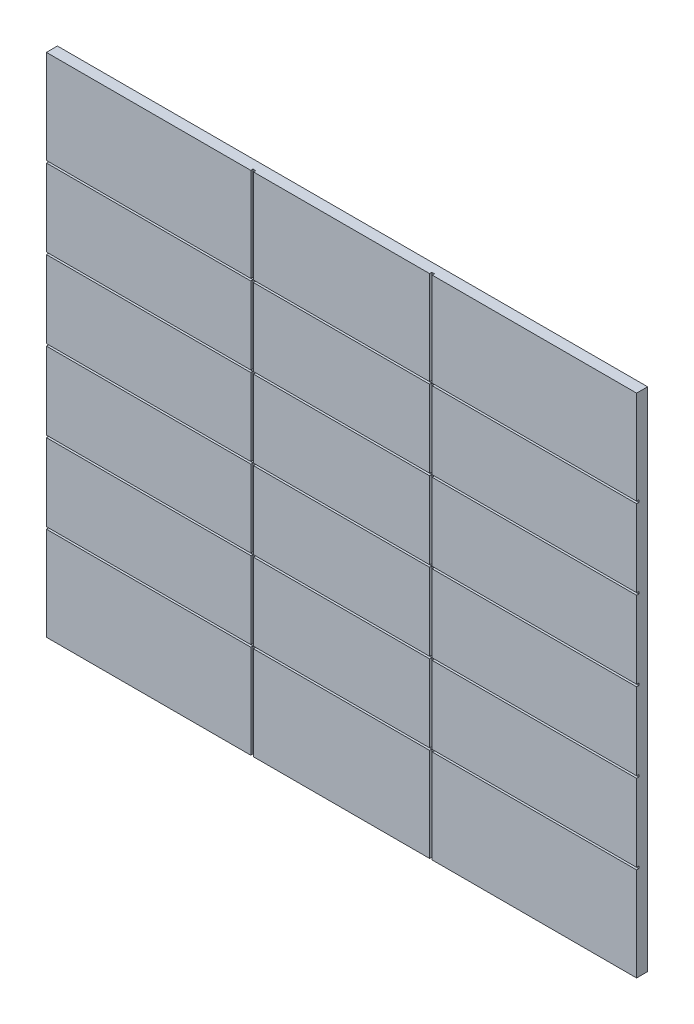
from build123d import *

# Parameters (mm, degrees)
SKETCH1_W           = 1340
SKETCH1_H           = 1150
BOSS_EXTRUDE1_DEPTH = 25
SKETCH2_W           = 1379.704401218
SKETCH2_H           = 5
CUT_EXTRUDE1_DEPTH  = 5
SKETCH3_W           = 6
SKETCH3_H           = 1155.334708323
CUT_EXTRUDE2_DEPTH  = 5
LPATTERN1_COUNT     = 3
LPATTERN1_PITCH     = 180
LPATTERN1_COL_COUNT = 3
LPATTERN1_COL_PITCH = 180
SWEEP1_PROFILE_R    = 5
SKETCH13_R          = 1.5
CUT_EXTRUDE3_DEPTH  = 10


with BuildPart() as part:
    # Sketch1 → Boss-Extrude1 (new body)
    with BuildSketch(Plane.XY):
        Rectangle(SKETCH1_W, SKETCH1_H)
    extrude(amount=BOSS_EXTRUDE1_DEPTH)

    # Sketch2 → Cut-Extrude1 (cut)
    with BuildSketch(Plane.XY.offset(25)):
        Rectangle(SKETCH2_W, SKETCH2_H)
    cut_extrude1 = extrude(amount=-CUT_EXTRUDE1_DEPTH, mode=Mode.SUBTRACT)

    # Sketch3 → Cut-Extrude2 (cut)
    with BuildSketch(Plane.XY.offset(25)):
        with Locations((203, -0.575515136)):
            Rectangle(SKETCH3_W, SKETCH3_H)
        with Locations((-203, -0.575515136)):
            Rectangle(SKETCH3_W, SKETCH3_H)
    extrude(amount=-CUT_EXTRUDE2_DEPTH, mode=Mode.SUBTRACT)

    # LPattern1: Cut-Extrude1 ×3
    with Locations(*[(0, -i * LPATTERN1_PITCH, 0) for i in range(1, LPATTERN1_COUNT)]):
        add(cut_extrude1, mode=Mode.SUBTRACT)

    # LPattern1 col: Cut-Extrude1 ×3
    with Locations(*[(0, i * LPATTERN1_COL_PITCH, 0) for i in range(1, LPATTERN1_COL_COUNT)]):
        add(cut_extrude1, mode=Mode.SUBTRACT)

    # Sweep1: sweep along a path in Sketch4
    with BuildLine(Plane(origin=(-49.523696958, -434, -370.281312655), x_dir=(0.9899494936611666, 0, -0.14142135623730917), z_dir=(0, -1, 0))) as sweep1_path:
        Line((362.941585957, 425.889408172), (367.184226644, 396.190923362))
    # Sweep1 profile (on start of the path) → Sweep1 (sweep)
    with BuildSketch(Plane(origin=(370, -434, 0), x_dir=(-1, 0, 0), z_dir=(0, 0, -1))):
        Circle(SWEEP1_PROFILE_R)
    sweep(path=sweep1_path.line)

    # Sketch13 → Cut-Extrude3 (cut)
    with BuildSketch(Plane(origin=(0, 0, -30), x_dir=(-1, 0, 0), z_dir=(0, 0, -1))):
        with Locations((-370, -434)):
            Circle(SKETCH13_R)
    extrude(amount=-CUT_EXTRUDE3_DEPTH, mode=Mode.SUBTRACT)


solid = part.part
